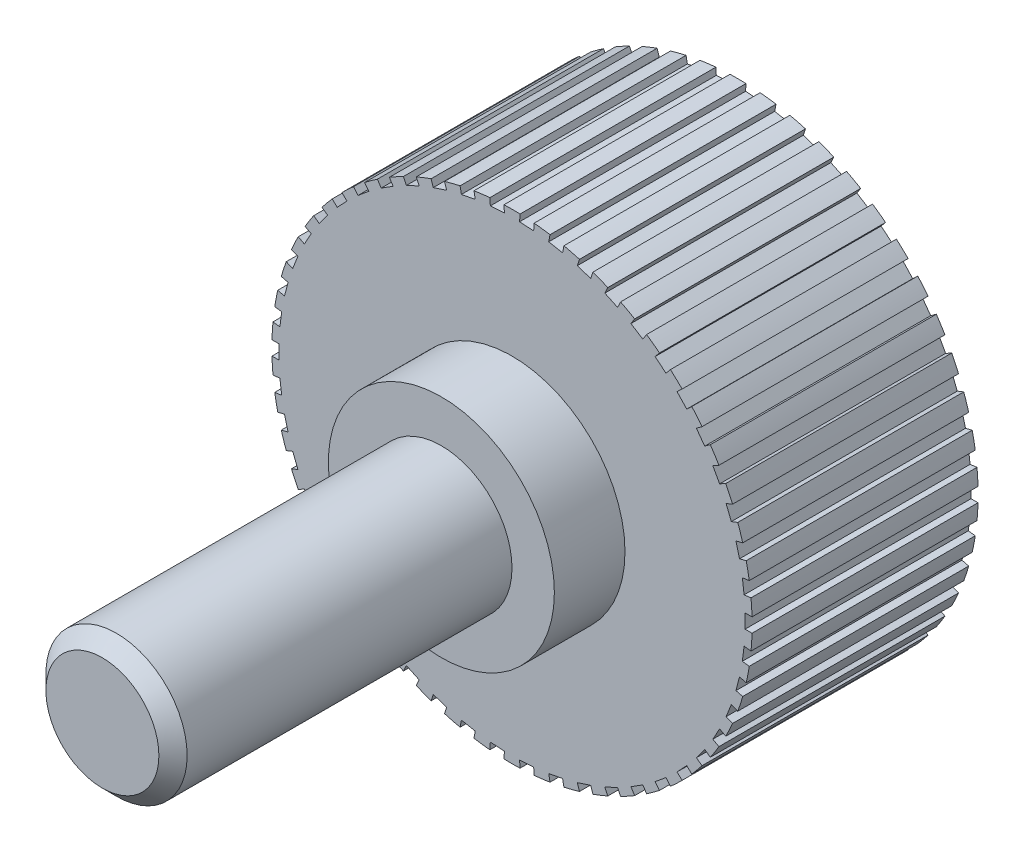
SolidWorks part; units mm, degrees
ref_plane "Front Plane" through (0, 0, 0) normal (0, 0, 1) x (1, 0, 0)
ref_plane "Top Plane" through (0, 0, 0) normal (0, 1, 0) x (1, 0, 0)
ref_plane "Right Plane" through (0, 0, 0) normal (1, 0, 0) x (0, 0, -1)
sketch "Sketch1" plane through (0, 0, 0) normal (0, 0, 1) x (1, 0, 0)
  circle A0 centre (0, 0) radius 8.5
  dimension "D1" = 17
extrude "Boss-Extrude1" add sketch "Sketch1" along normal blind 8
sketch "Sketch2" plane through (0, 0, 8) normal (0, 0, 1) x (1, 0, 0)
  circle A0 centre (0, 0) radius 4
  dimension "D1" = 8
extrude "Boss-Extrude2" add sketch "Sketch2" along normal blind 2.5
sketch "Sketch3" plane through (0, 0, 10.5) normal (0, 0, 1) x (1, 0, 0)
  circle A0 centre (0, 0) radius 2.5
  dimension "D1" = 5
extrude "Boss-Extrude3" add sketch "Sketch3" along normal blind 12
cosmetic thread "Cosmetic Thread1" parameters "D1"=10, "D2"=4.134
chamfer "Chamfer1" distance 0.5 angle 45 1 edges at (2.5, 0, 22.5)
sketch "Sketch5" plane through (0, 0, 8) normal (0, 0, 1) x (1, 0, 0)
  line L0 (0, 0) -> (11.8016, 0) construction
  line L2 (8.25, 0.25) -> (8.75, 0.25)
  line L3 (8.25, 0.25) -> (8.25, -0.25)
  line L4 (8.25, -0.25) -> (8.75, -0.25)
  line L5 (8.75, 0.25) -> (8.75, -0.25)
  line L6 (8.25, 0.25) -> (8.75, -0.25) construction
  line L7 (8.25, -0.25) -> (8.75, 0.25) construction
  circle A1 centre (0, 0) radius 8.5 construction
  point P2 (8.5, 0)
  dimension "D1" = 0.5
  dimension "D2" = 0.5
extrude "Cut-Extrude2" cut sketch "Sketch5" against normal blind 10
pattern_circular "CirPattern2" count 50 over 360 about axis through (0, 0, 0) along (0, 0, 1) of "Cut-Extrude2"
